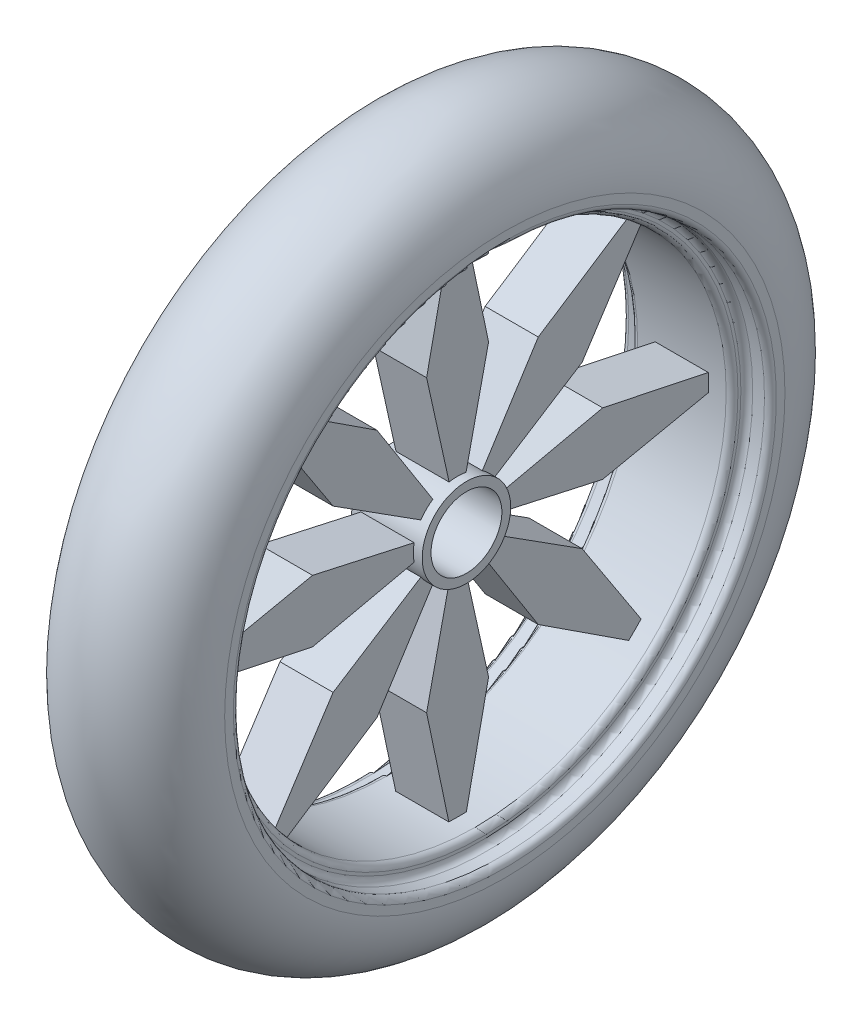
SolidWorks part; units mm, degrees
ref_plane "Front Plane" through (0, 0, 0) normal (0, 0, 1) x (1, 0, 0)
ref_plane "Top Plane" through (0, 0, 0) normal (0, 1, 0) x (1, 0, 0)
ref_plane "Right Plane" through (0, 0, 0) normal (1, 0, 0) x (0, 0, -1)
other "Configuration Table"
sketch "Sketch1" plane through (0, 0, 0) normal (0, 0, 1) x (1, 0, 0)
  line L0 (0, 0) -> (0, 62.8322) construction
  line L1 (25, 94.9309) -> (25, 90)
  line L2 (25, 90) -> (-25, 90)
  line L3 (-25, 90) -> (-25, 94.9309)
  line L4 (0, 0) -> (47.0772, 0) construction
  arc A0 (-25, 94.9309) -> (25, 94.9309) centre (0, 94.9309) cw
  dimension "D1" = 25
  dimension "D2" = 90
revolve "Revolve1" add sketch "Sketch1" angle 360 about L4
sketch "Sketch2" plane through (0, 0, 0) normal (1, 0, 0) x (0, 0, -1)
  circle A0 centre (0, 0) radius 90
  circle A1 centre (0, 0) radius 85
  dimension "D1" = 180
  dimension "D2" = 170
extrude "Boss-Extrude1" add sketch "Sketch2" along normal mid plane 34 contours A0
sketch "Sketch3" plane through (0, 0, 0) normal (1, 0, 0) x (0, 0, -1)
  circle A0 centre (0, 0) radius 15
  circle A1 centre (0, 0) radius 12
  dimension "D1" = 30
  dimension "D2" = 24
extrude "Boss-Extrude2" add sketch "Sketch3" along normal mid plane 24 separate body
fillet "Fillet1" radius 2 6 edges at (17, 0, -85) (-17, 0, -85) (17, 0, -90) (-17, 0, -90) (-25, 0, 90) (25, 0, 90)
sketch "Sketch4" plane through (0, 0, 0) normal (1, 0, 0) x (0, 0, -1)
  line L0 (-2.5528, 86.9625) -> (-10.4973, 49.1563)
  line L1 (-10.4973, 49.1563) -> (-2.5234, 13.1699)
  line L2 (0, 0) -> (0, 103.6081) construction
  line L3 (10.4973, 49.1563) -> (2.5234, 13.1699)
  line L4 (2.5528, 86.9625) -> (10.4973, 49.1563)
  line L5 (-2.5528, 86.9625) -> (2.5528, 86.9625)
  line L6 (2.5234, 13.1699) -> (-2.5234, 13.1699)
  circle A0 centre (0, 0) radius 87 construction
extrude "Boss-Extrude3" add sketch "Sketch4" along normal mid plane 18
pattern_circular "CirPattern1" count 8 over 360 about axis through (0, 0, 0) along (1, 0, 0) of "Boss-Extrude3"
